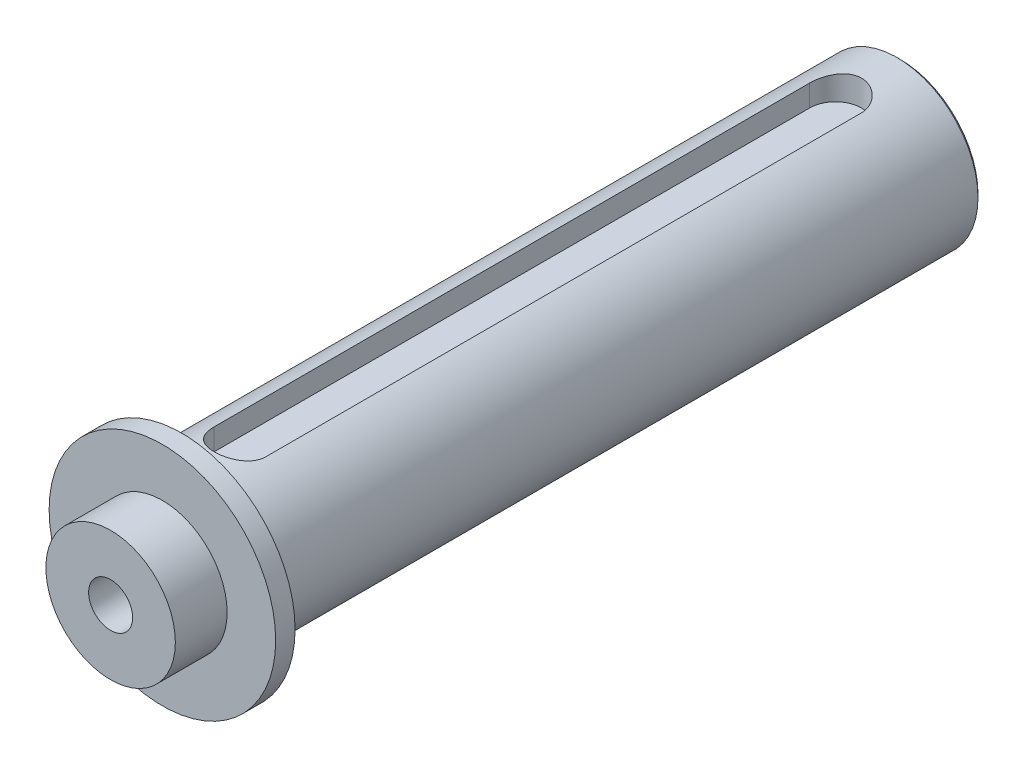
from build123d import *

# Parameters (mm, degrees)
SKETCH_1_R              = 12.5
EXTRUDE_1_DEPTH         = 111
SKETCH_2_R              = 17.5
EXTRUDE_2_DEPTH         = 3
SKETCH_3_R              = 10
EXTRUDE_3_DEPTH         = 8
CUT_EXTRUDE_1_DEPTH     = 4
HOLE_WIZARD_M8_1_D      = 6.8
HOLE_WIZARD_M8_1_DEPTH  = 23.75
HOLE_WIZARD_M8_1_TIP    = 2.042926105
HOLE_WIZARD_M12_1_D     = 10.2
HOLE_WIZARD_M12_1_DEPTH = 30.25
HOLE_WIZARD_M12_1_TIP   = 3.064389157
CHAMFER_1_SIZE          = 0.5


with BuildPart() as part:
    # 草图1 → 凸台-拉伸1 (new body)
    with BuildSketch(Plane.XY):
        Circle(SKETCH_1_R)
    extrude(amount=EXTRUDE_1_DEPTH)

    # 草图2 → 凸台-拉伸2 (add)
    with BuildSketch(Plane.XY.offset(111)):
        Circle(SKETCH_2_R)
    extrude(amount=EXTRUDE_2_DEPTH)

    # 草图3 → 凸台-拉伸3 (add)
    with BuildSketch(Plane.XY.offset(114)):
        Circle(SKETCH_3_R)
    extrude(amount=EXTRUDE_3_DEPTH)

    # 草图4 → 切除-拉伸1 (cut)
    with BuildSketch(Plane(origin=(0, 12.5, 0), x_dir=(1, 0, 0), z_dir=(0, 1, 0))):
        with BuildLine():
            Line((4, -10), (4, -102))
            ThreePointArc((4, -102), (0, -106), (-4, -102))
            Line((-4, -102), (-4, -10))
            ThreePointArc((-4, -10), (0, -6), (4, -10))
        make_face()
    extrude(amount=-CUT_EXTRUDE_1_DEPTH, mode=Mode.SUBTRACT)

    # M8 螺纹孔1
    with Locations(Plane.XY.offset(122)):
        with Locations((0, 0)):
            Hole(HOLE_WIZARD_M8_1_D / 2, depth=HOLE_WIZARD_M8_1_DEPTH)
            with Locations((0, 0, -(HOLE_WIZARD_M8_1_DEPTH + HOLE_WIZARD_M8_1_TIP / 2))):  # 118° drill point
                Cone(0, HOLE_WIZARD_M8_1_D / 2, HOLE_WIZARD_M8_1_TIP, mode=Mode.SUBTRACT)

    # M12 螺纹孔1
    with Locations(Plane(origin=(0, 0, 0), x_dir=(-1, 0, 0), z_dir=(0, 0, -1))):
        with Locations((0, 0)):
            Hole(HOLE_WIZARD_M12_1_D / 2, depth=HOLE_WIZARD_M12_1_DEPTH)
            with Locations((0, 0, -(HOLE_WIZARD_M12_1_DEPTH + HOLE_WIZARD_M12_1_TIP / 2))):  # 118° drill point
                Cone(0, HOLE_WIZARD_M12_1_D / 2, HOLE_WIZARD_M12_1_TIP, mode=Mode.SUBTRACT)

    # 倒角1
    chamfer_1_edges = [part.edges().sort_by_distance(p)[0] for p in [
        (-12.5, 0, 0),
    ]]
    chamfer(chamfer_1_edges, length=CHAMFER_1_SIZE)


solid = part.part
